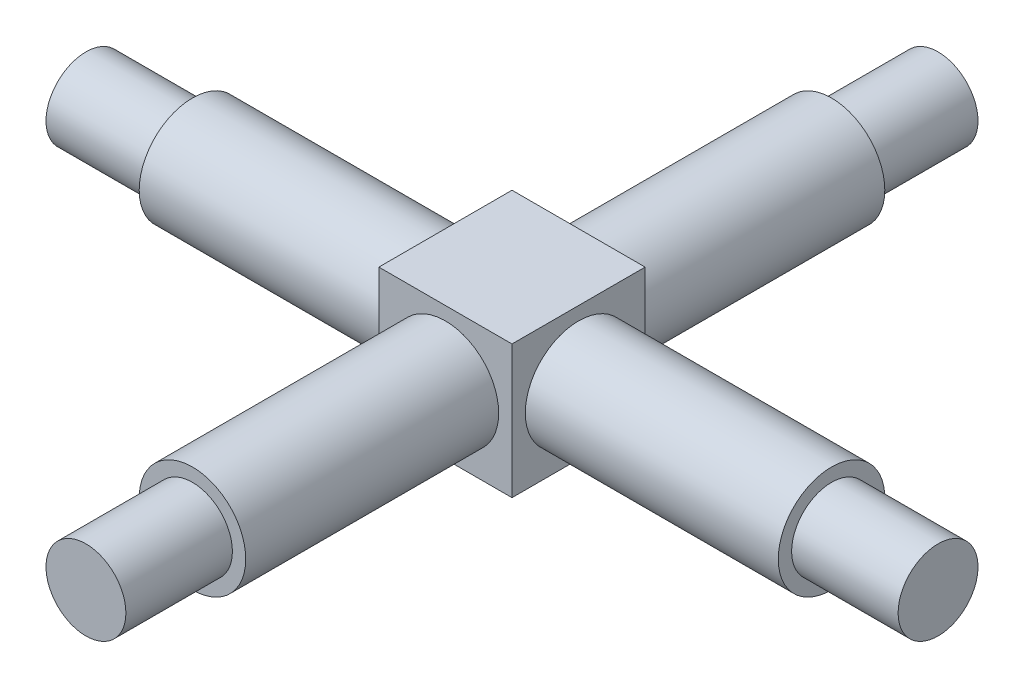
from build123d import *

# Parameters (mm, degrees)
SKETCH1_W           = 5
SKETCH1_H           = 5
BOSS_EXTRUDE1_DEPTH = 5
SKETCH2_R           = 2
BOSS_EXTRUDE2_DEPTH = 13.5
SKETCH3_R           = 2
BOSS_EXTRUDE3_DEPTH = 13.5
SKETCH4_R           = 2
SKETCH4_R_2         = 1.5
CUT_EXTRUDE1_DEPTH  = 4
SKETCH5_R           = 2
SKETCH5_R_2         = 1.5
CUT_EXTRUDE2_DEPTH  = 4


with BuildPart() as part:
    # Sketch1 → Boss-Extrude1 (new body)
    with BuildSketch(Plane.XY):
        with Locations((-28.193643968, 28.298971706)):
            Rectangle(SKETCH1_W, SKETCH1_H)
    extrude(amount=BOSS_EXTRUDE1_DEPTH)

    # Sketch2 → Boss-Extrude2 (add)
    with BuildSketch(Plane.XY.offset(5)):
        with Locations((-28.193643968, 28.298971706)):
            Circle(SKETCH2_R)
    boss_extrude2 = extrude(amount=BOSS_EXTRUDE2_DEPTH)

    # Sketch3 → Boss-Extrude3 (add)
    with BuildSketch(Plane(origin=(-25.693643968, 0, 0), x_dir=(0, 0, -1), z_dir=(1, 0, 0))):
        with Locations((-2.5, 28.298971706)):
            Circle(SKETCH3_R)
    boss_extrude3 = extrude(amount=BOSS_EXTRUDE3_DEPTH)

    # Mirror1: Boss-Extrude2 across plane
    add(boss_extrude2.mirror(Plane(origin=(0, 0, 2.5), x_dir=(1, 0, 0), z_dir=(0, 0, -1))))

    # Mirror2: Boss-Extrude3 across plane
    add(boss_extrude3.mirror(Plane(origin=(-28.193643968, 0, 0), x_dir=(0, 0, 1), z_dir=(1, 0, 0))))

    # Sketch4 → Cut-Extrude1 (cut)
    with BuildSketch(Plane.XY.offset(18.5)):
        with Locations((-28.193643968, 28.298971706)):
            Circle(SKETCH4_R)
        with Locations((-28.193643968, 28.298971706)):
            Circle(SKETCH4_R_2, mode=Mode.SUBTRACT)
    cut_extrude1 = extrude(amount=-CUT_EXTRUDE1_DEPTH, mode=Mode.SUBTRACT)

    # Mirror3: Cut-Extrude1 across plane
    add(cut_extrude1.mirror(Plane(origin=(0, 0, 2.5), x_dir=(1, 0, 0), z_dir=(0, 0, -1))), mode=Mode.SUBTRACT)

    # Sketch5 → Cut-Extrude2 (cut)
    with BuildSketch(Plane.ZY.offset(44.193643968)):
        with Locations(Location((2.5, 28.298971706, 0), (0, 0, 180))):
            Circle(SKETCH5_R)
        with Locations((2.5, 28.298971706)):
            Circle(SKETCH5_R_2, mode=Mode.SUBTRACT)
    cut_extrude2 = extrude(amount=-CUT_EXTRUDE2_DEPTH, mode=Mode.SUBTRACT)

    # Mirror4: Cut-Extrude2 across plane
    add(cut_extrude2.mirror(Plane(origin=(-28.193643968, 0, 0), x_dir=(0, 0, 1), z_dir=(1, 0, 0))), mode=Mode.SUBTRACT)


solid = part.part
